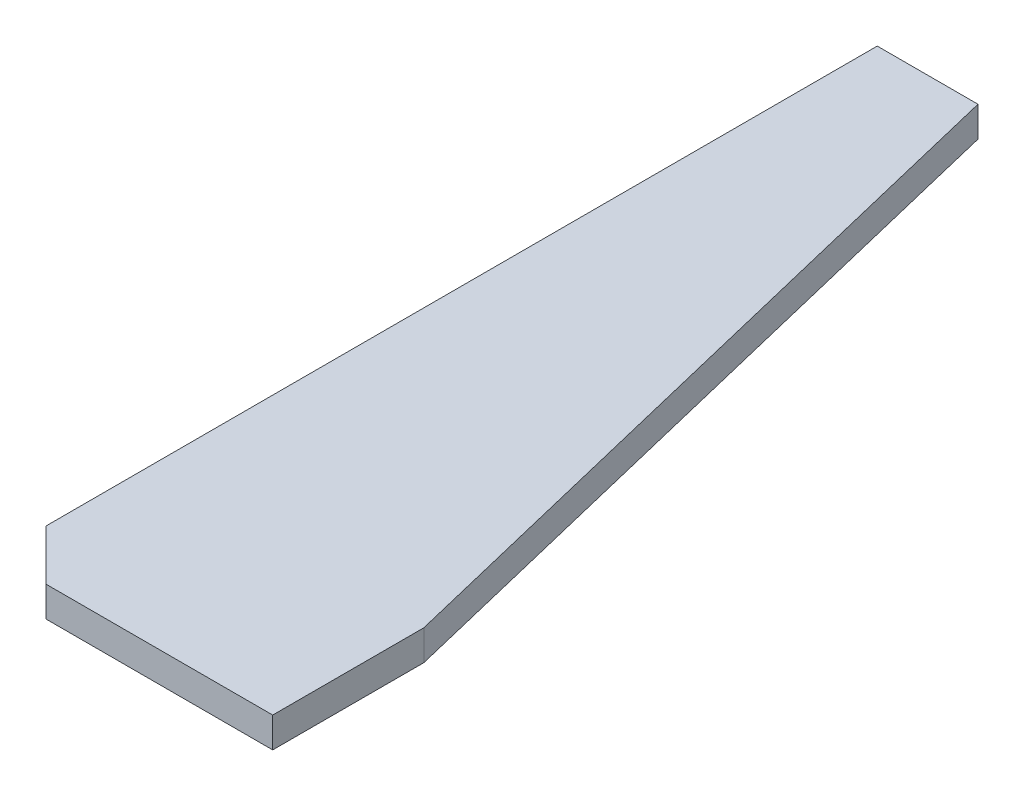
from build123d import *

# Parameters (mm, degrees)
BOSS_EXTRUDE1_DEPTH = 6
CHAMFER1_SIZE       = 20


with BuildPart() as part:
    # Sketch1 → Boss-Extrude1 (new, symmetric)
    with BuildSketch(Plane(origin=(0, 0, 0), x_dir=(1, 0, 0), z_dir=(0, 1, 0))):
        Polygon((-20, 20), (-20, 350), (20, 350), (90, 60), (90, 0), (0, 0), (-20, 0), align=None)
    extrude(amount=BOSS_EXTRUDE1_DEPTH, both=True)

    # Chamfer1
    chamfer1_edges = [part.edges().sort_by_distance(p)[0] for p in [
        (-20, 0, 0),
    ]]
    chamfer(chamfer1_edges, length=CHAMFER1_SIZE)


solid = part.part
